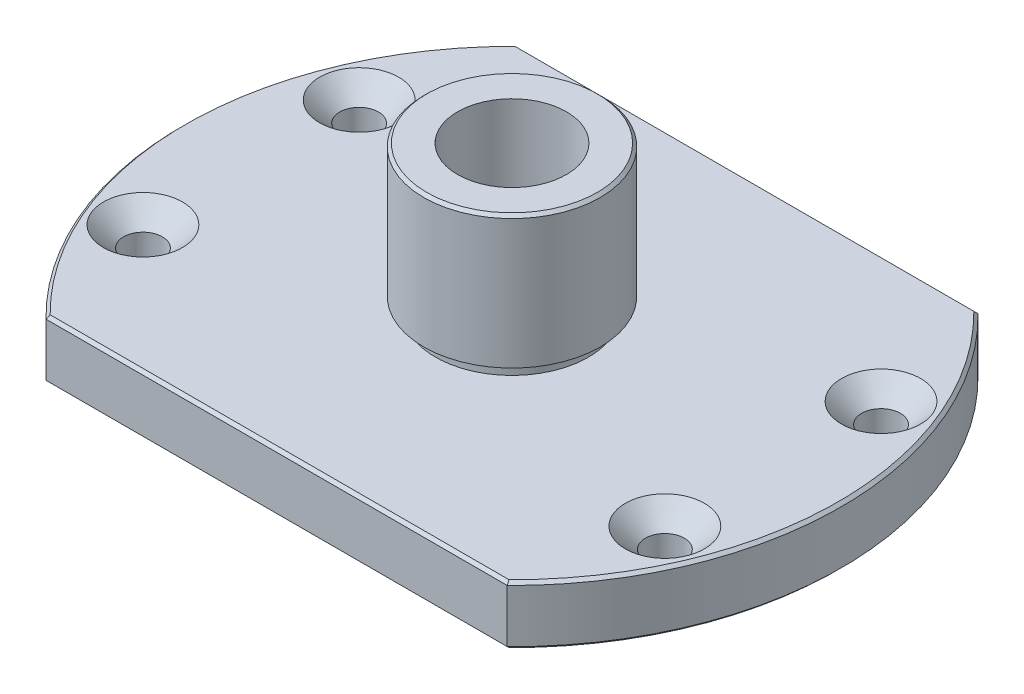
from build123d import *

# Parameters (mm, degrees)
SKETCH_1_R                   = 56
EXTRUDE_1_DEPTH              = 10
SKETCH_2_R                   = 15
EXTRUDE_2_DEPTH              = 25
M20X1_5_1_D                  = 18.5
M20X1_5_1_DEPTH              = 44.5
M20X1_5_1_TIP                = 5.557960726
HOLE_WIZARD_M6_1_D           = 6.6
HOLE_WIZARD_M6_1_CSINK_D     = 13.44
HOLE_WIZARD_M6_1_CSINK_ANGLE = 90
SKETCH_12_OUTSIDE_W          = 146.442
SKETCH_12_OUTSIDE_H          = 146.442
SKETCH_12_OUTSIDE_W_2        = 136.125327254
SKETCH_12_OUTSIDE_H_2        = 80
CUT_EXTRUDE_1_DEPTH          = 25
SKETCH_13_W                  = 2
SKETCH_13_H                  = 2.5
CHAMFER_7_SIZE               = 0.5
SKETCH_14_R                  = 15
CUT_EXTRUDE_2_DEPTH          = 5


with BuildPart() as part:
    # 草图1 → 凸台-拉伸1 (new body)
    with BuildSketch(Plane(origin=(0, 0, 0), x_dir=(1, 0, 0), z_dir=(0, 1, 0))):
        with Locations(Location((0, 0, 0), (0, 0, 270))):
            Circle(SKETCH_1_R)
    extrude(amount=EXTRUDE_1_DEPTH)

    # 草图2 → 凸台-拉伸2 (add)
    with BuildSketch(Plane(origin=(0, 10, 0), x_dir=(1, 0, 0), z_dir=(0, 1, 0))):
        with Locations(Location((0, 0, 0), (0, 0, 270))):
            Circle(SKETCH_2_R)
    extrude(amount=EXTRUDE_2_DEPTH)

    # M20x1.5 螺纹孔1
    with Locations(Plane(origin=(0, 35, 0), x_dir=(1, 0, 0), z_dir=(0, 1, 0))):
        with Locations((0, 0)):
            Hole(M20X1_5_1_D / 2, depth=M20X1_5_1_DEPTH)
            with Locations((0, 0, -(M20X1_5_1_DEPTH + M20X1_5_1_TIP / 2))):  # 118° drill point
                Cone(0, M20X1_5_1_D / 2, M20X1_5_1_TIP, mode=Mode.SUBTRACT)

    # M6 六角凹锥坑螺钉的锥形沉头孔1 (through all)
    with Locations(Plane(origin=(0, 10, 0), x_dir=(1, 0, 0), z_dir=(0, 1, 0))):
        with Locations((44.346217561, -18.368804754), (-44.346217561, 18.368804754), (-44.346217561, -18.368804754), (44.346217561, 18.368804754)):
            CounterSinkHole(HOLE_WIZARD_M6_1_D / 2, HOLE_WIZARD_M6_1_CSINK_D / 2, counter_sink_angle=HOLE_WIZARD_M6_1_CSINK_ANGLE)

    # 草图12 outside → 切除-拉伸1 (cut)
    with BuildSketch(Plane(origin=(0, 10, 0), x_dir=(1, 0, 0), z_dir=(0, 1, 0))):
        Rectangle(SKETCH_12_OUTSIDE_W, SKETCH_12_OUTSIDE_H)
        Rectangle(SKETCH_12_OUTSIDE_W_2, SKETCH_12_OUTSIDE_H_2, mode=Mode.SUBTRACT)
    extrude(amount=-CUT_EXTRUDE_1_DEPTH, mode=Mode.SUBTRACT)

    # 草图13 → 切除-旋转1 (revolve, cut)
    with BuildSketch(Plane.XY, mode=Mode.PRIVATE) as cut_revolve_1_sk:
        with Locations((-14, 11.25)):
            Rectangle(SKETCH_13_W, SKETCH_13_H)
    revolve(cut_revolve_1_sk.sketch.rotate(Axis((0, -2.79729943, 0), (0, 1, 0)), 270), axis=Axis((0, -2.79729943, 0), (0, 1, 0)), mode=Mode.SUBTRACT)

    # 倒角7
    chamfer_7_edges = [part.edges().sort_by_distance(p)[0] for p in [
        (56, 0, 0),
        (56, 10, 0),
        (-56, 0, 0),
        (0, 0, -40),
        (0, 0, 40),
        (-56, 10, 0),
        (0, 10, 40),
        (0, 10, -40),
        (0, 35, -15),
    ]]
    chamfer(chamfer_7_edges, length=CHAMFER_7_SIZE)

    # 草图14 → 切除-拉伸2 (cut)
    with BuildSketch(Plane.XZ):
        with Locations(Location((0, 0, 0), (0, 0, 270))):
            Circle(SKETCH_14_R)
    extrude(amount=-CUT_EXTRUDE_2_DEPTH, mode=Mode.SUBTRACT)


solid = part.part
